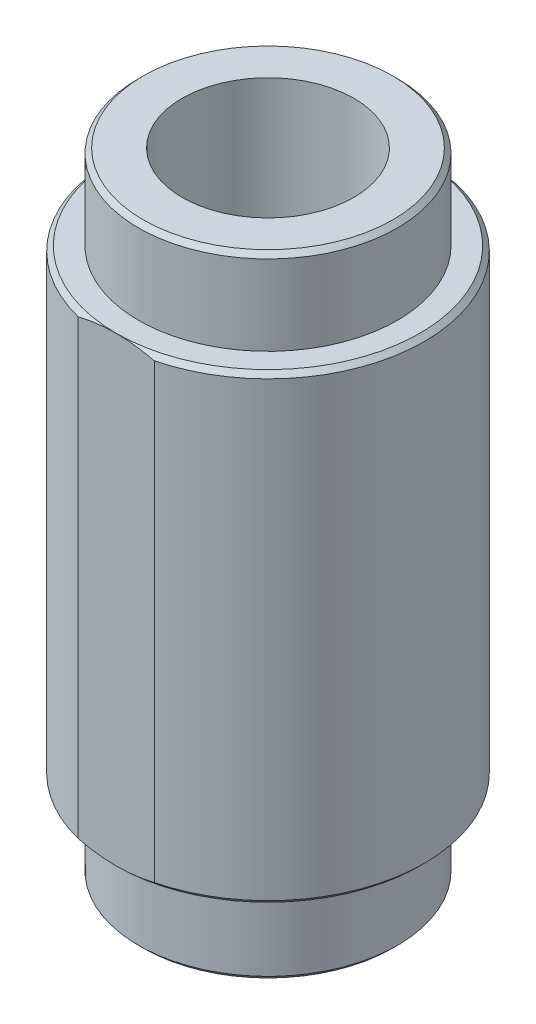
from build123d import *

# Parameters (mm, degrees)
CUT_EXTRUDE1_DEPTH = 251.336773168


with BuildPart() as part:
    # Sketch1 → Revolve1 (revolve)
    with BuildSketch(Plane.XY, mode=Mode.PRIVATE) as revolve1_sk:
        Polygon((-66.5, 230), (-66.5, 38), (-64.5, 36), (-55, 36), (-55, 2), (-53, 0), (-36.5, 0), (-36.5, 268), (-53, 268), (-55, 266), (-55, 232), (-64.5, 232), align=None)
    revolve(revolve1_sk.sketch.rotate(Axis((0, -26.656454657, 0), (0, 1, 0)), 270), axis=Axis((0, -26.656454657, 0), (0, 1, 0)))

    # Sketch2 → Cut-Extrude1 (cut, through all)
    with BuildSketch(Plane.XZ.offset(-36)):
        with BuildLine():
            Line((-16.186414056, 64.5), (16.186414056, 64.5))
            ThreePointArc((16.186414056, 64.5), (0, 66.5), (-16.186414056, 64.5))
        make_face()
        with BuildLine():
            Line((-16.186414056, -64.5), (16.186414056, -64.5))
            ThreePointArc((16.186414056, -64.5), (0, -66.5), (-16.186414056, -64.5))
        make_face()
    extrude(amount=-CUT_EXTRUDE1_DEPTH, mode=Mode.SUBTRACT)


solid = part.part
